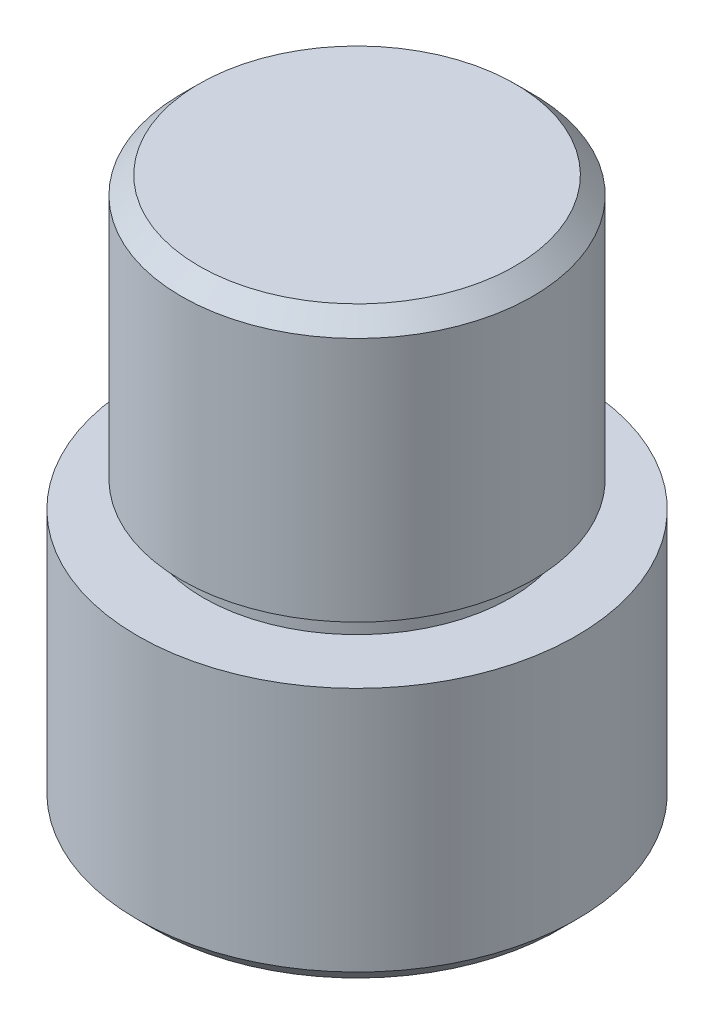
SolidWorks part; units mm, degrees
ref_plane "Front Plane" through (0, 0, 0) normal (0, 0, 1) x (1, 0, 0)
ref_plane "Top Plane" through (0, 0, 0) normal (0, 1, 0) x (1, 0, 0)
ref_plane "Right Plane" through (0, 0, 0) normal (1, 0, 0) x (0, 0, -1)
sketch "Sketch1" plane through (0, 0, 0) normal (0, 0, 1) x (1, 0, 0)
  line L0 (0, 37.5) -> (0, -34.5) construction
  line L2 (0, 27.3947) -> (-20, 27.3947)
  line L3 (0, 27.3947) -> (0, -2.6053)
  line L4 (0, -2.6053) -> (-20, -2.6053)
  line L5 (-20, 27.3947) -> (-20, -2.6053)
  line L6 (0, -2.6053) -> (-17.5, -2.6053)
  line L7 (0, -2.6053) -> (0, -5.6053)
  line L8 (0, -5.6053) -> (-17.5, -5.6053)
  line L9 (-17.5, -2.6053) -> (-17.5, -5.6053)
  line L10 (0, -5.6053) -> (-25, -5.6053)
  line L11 (0, -5.6053) -> (0, -35.6053)
  line L12 (0, -35.6053) -> (-25, -35.6053)
  line L13 (-25, -5.6053) -> (-25, -35.6053)
  dimension "D1" = 30
  dimension "D2" = 20
  dimension "D3" = 3
  dimension "D4" = 17.5
  dimension "D5" = 25
  dimension "D6" = 30
revolve "Revolve1" add sketch "Sketch1" angle 360 about L0
chamfer "Chamfer1" distance 2 angle 45 1 edges at (0, 27.3947, 20)
chamfer "Chamfer2" distance 2 angle 45 1 edges at (0, -35.6053, 25)
